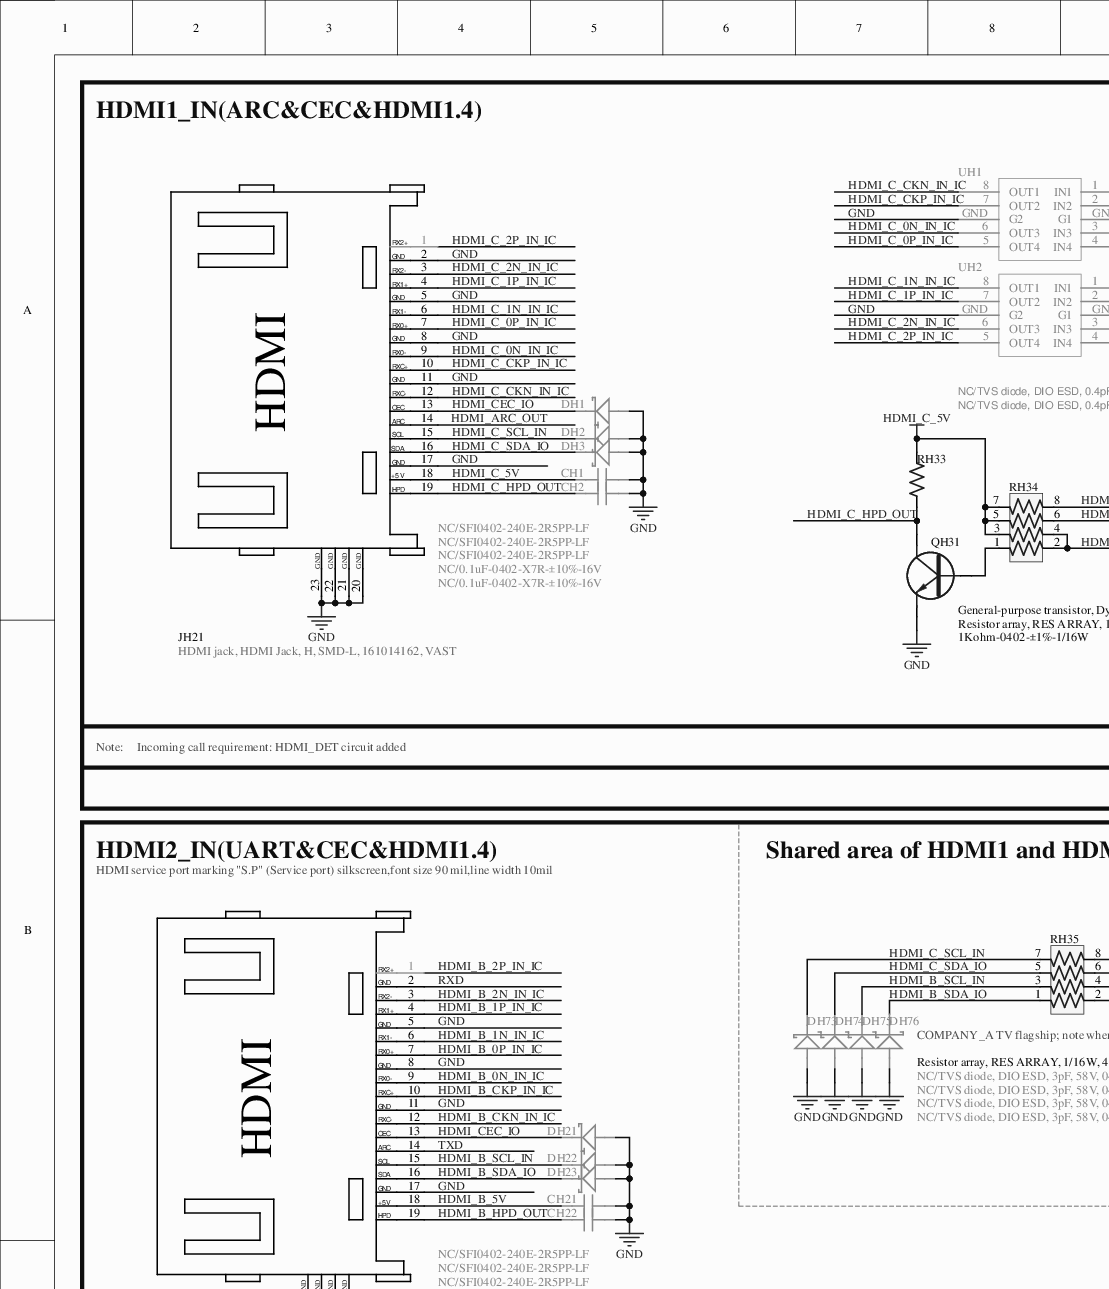
[diagram p0: MISC105950-40.SchDoc, top left]
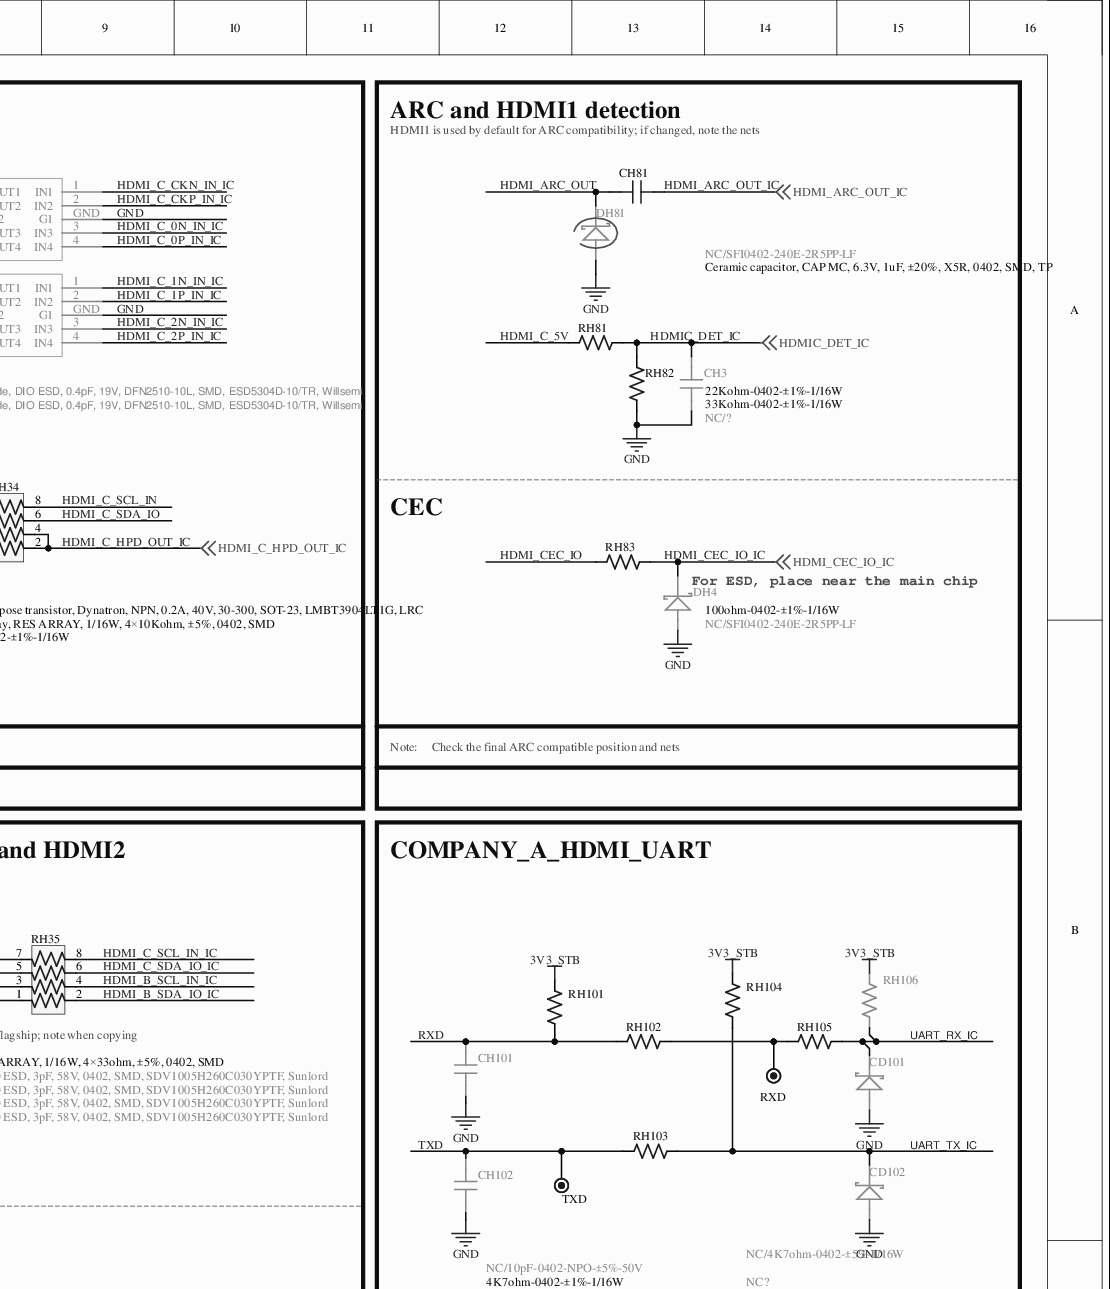
[diagram p1: MISC105950-40.SchDoc, top right]
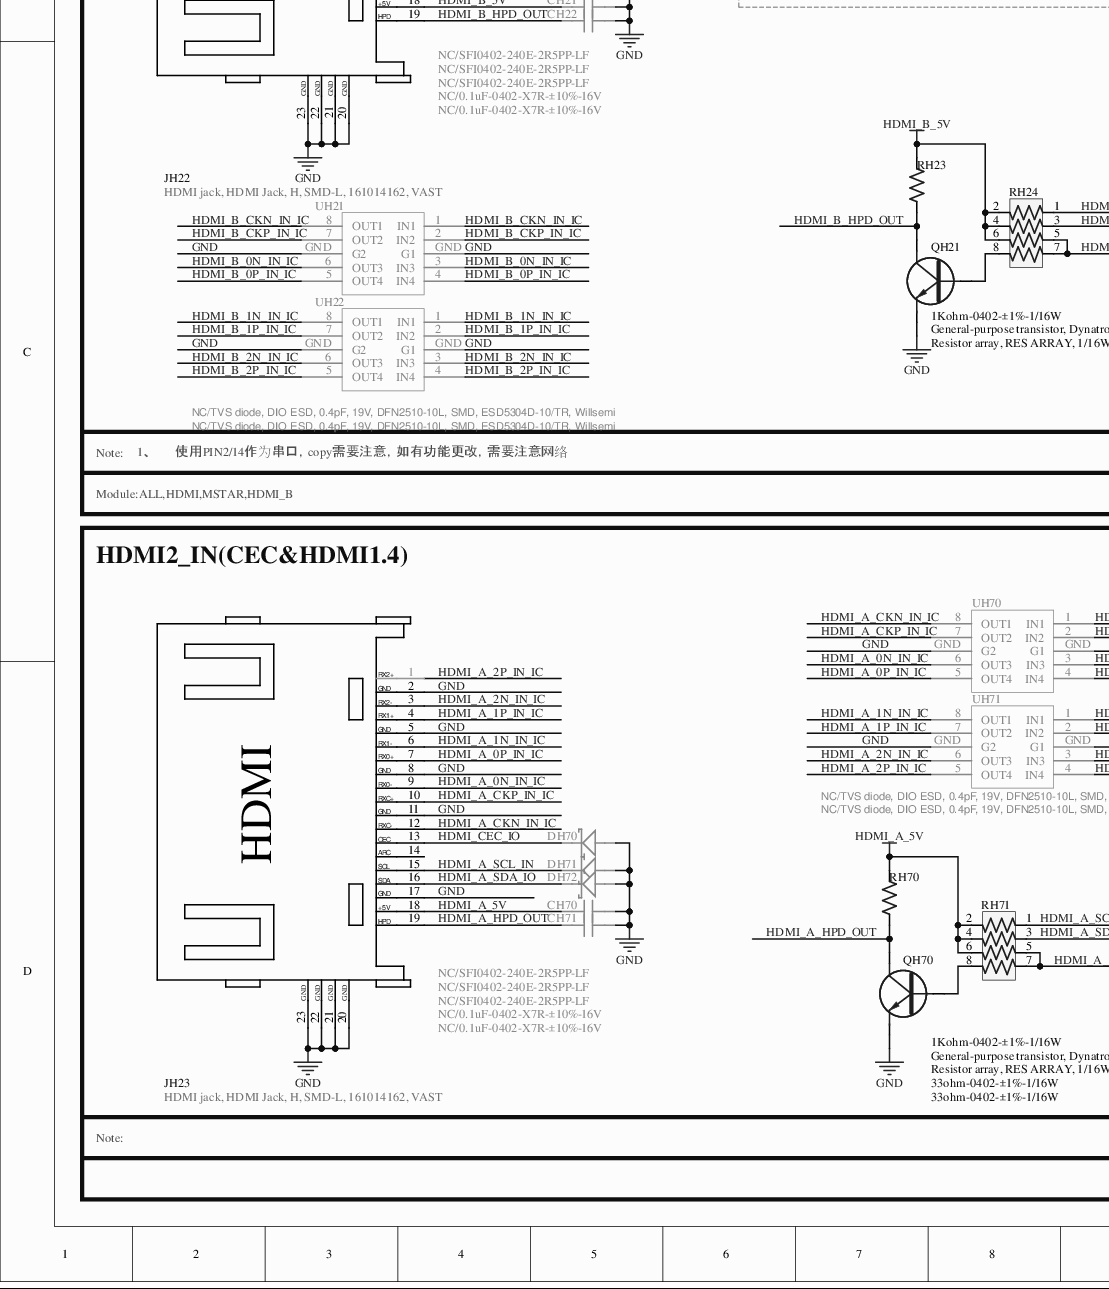
[diagram p2: MISC105950-40.SchDoc, bottom left]
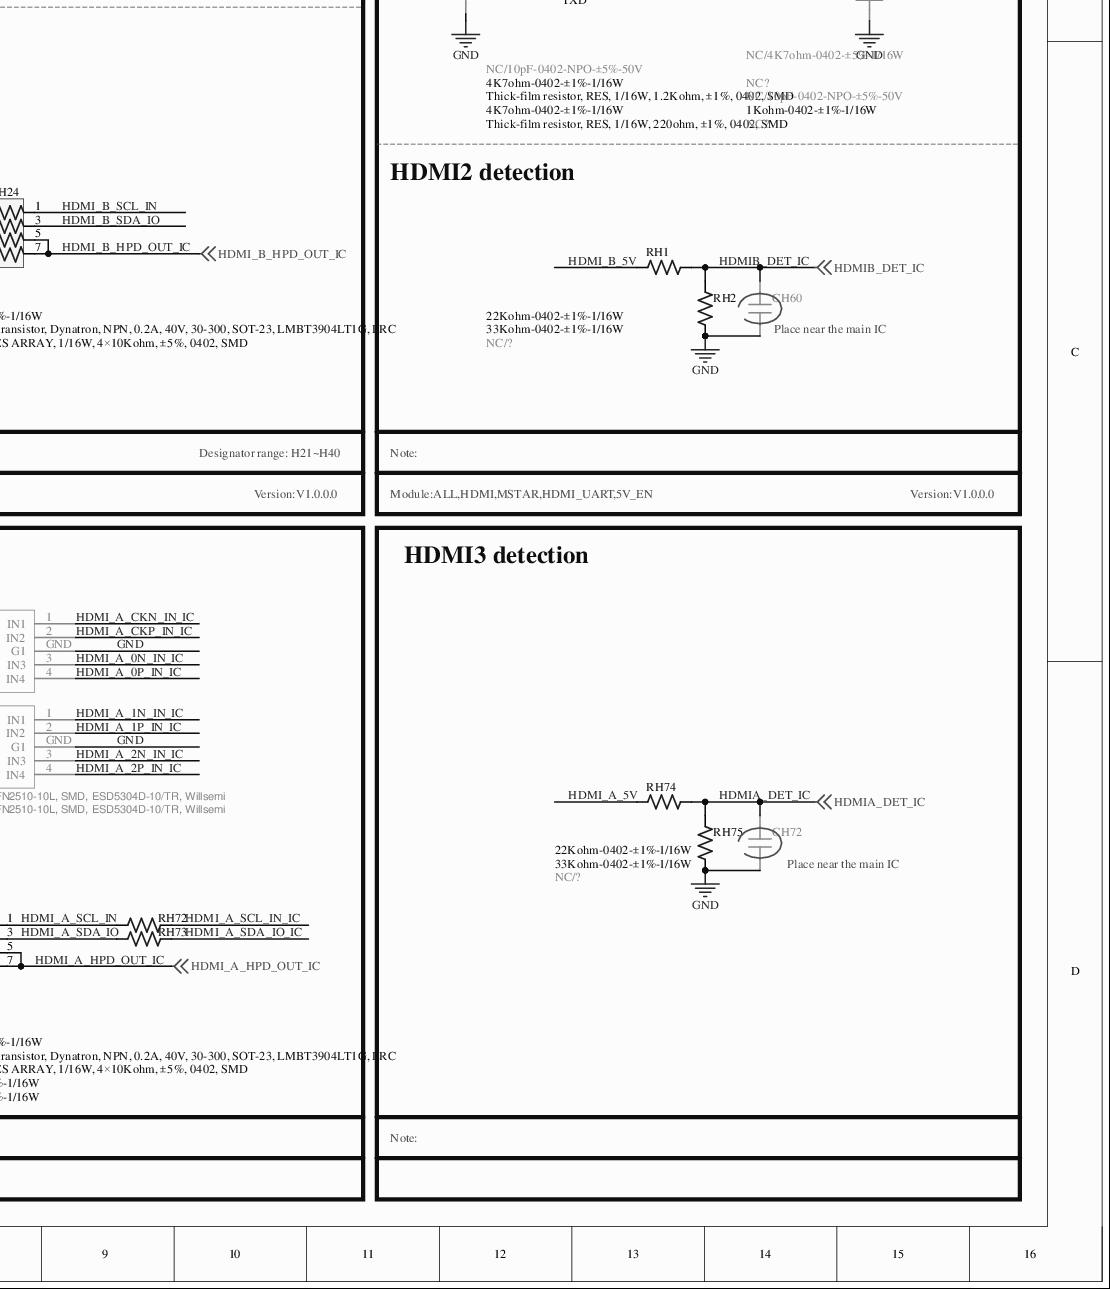
[diagram p3: MISC105950-40.SchDoc, bottom right]
# Altium project MISC105950-48.PrjPCB (part 6 of 8)

## Sheet MISC105950-40.SchDoc
size 393 x 459 mm

### Parts
CD101  NC?  [DIODE-S0402]
CD102  NC?  [DIODE-S0402]
CH1  NC/0.1uF-0402-X7R-±10%-16V  [C0402]
CH2  NC/0.1uF-0402-X7R-±10%-16V  [C0402]
CH3  NC/?  [C0402]
CH21  NC/0.1uF-0402-X7R-±10%-16V  [C0402]
CH22  NC/0.1uF-0402-X7R-±10%-16V  [C0402]
CH60  NC/?  [C0402]
CH70  NC/0.1uF-0402-X7R-±10%-16V  [C0402]
CH71  NC/0.1uF-0402-X7R-±10%-16V  [C0402]
CH72  NC/?  [C0402]
CH81  Ceramic capacitor, CAP MC, 6.3V, 1uF, ±20%, X5R, 0402, SMD, TP  [C0402]
CH101  NC/10pF-0402-NPO-±5%-50V  [C0402]
CH102  NC/10pF-0402-NPO-±5%-50V  [C0402]
DH1  NC/SFI0402-240E-2R5PP-LF  [DIODE-S0402]
DH2  NC/SFI0402-240E-2R5PP-LF  [DIODE-S0402]
DH3  NC/SFI0402-240E-2R5PP-LF  [DIODE-S0402]
DH4  NC/SFI0402-240E-2R5PP-LF  [DIODE-S0402]
DH21  NC/SFI0402-240E-2R5PP-LF  [DIODE-S0402]
DH22  NC/SFI0402-240E-2R5PP-LF  [DIODE-S0402]
DH23  NC/SFI0402-240E-2R5PP-LF  [DIODE-S0402]
DH70  NC/SFI0402-240E-2R5PP-LF  [DIODE-S0402]
DH71  NC/SFI0402-240E-2R5PP-LF  [DIODE-S0402]
DH72  NC/SFI0402-240E-2R5PP-LF  [DIODE-S0402]
DH73  NC/TVS diode, DIO ESD, 3pF, 58V, 0402, SMD, SDV1005H260C030YPTF, Sunlord  [DIODE-S0402]
DH74  NC/TVS diode, DIO ESD, 3pF, 58V, 0402, SMD, SDV1005H260C030YPTF, Sunlord  [DIODE-S0402]
DH75  NC/TVS diode, DIO ESD, 3pF, 58V, 0402, SMD, SDV1005H260C030YPTF, Sunlord  [DIODE-S0402]
DH76  NC/TVS diode, DIO ESD, 3pF, 58V, 0402, SMD, SDV1005H260C030YPTF, Sunlord  [DIODE-S0402]
DH81  NC/SFI0402-240E-2R5PP-LF  [DIODE-S0402]
JH21  HDMI jack, HDMI Jack, H, SMD-L, 161014162, VAST  [HDMI-HS-1]
JH22  HDMI jack, HDMI Jack, H, SMD-L, 161014162, VAST  [HDMI-HS-1]
JH23  HDMI jack, HDMI Jack, H, SMD-L, 161014162, VAST  [HDMI-HS-1]
QH21  General-purpose transistor, Dynatron, NPN, 0.2A, 40V, 30-300, SOT-23, LMBT3904LT1G, LRC  [SOT-23]
QH31  General-purpose transistor, Dynatron, NPN, 0.2A, 40V, 30-300, SOT-23, LMBT3904LT1G, LRC  [SOT-23]
QH70  General-purpose transistor, Dynatron, NPN, 0.2A, 40V, 30-300, SOT-23, LMBT3904LT1G, LRC  [SOT-23]
RH1  22Kohm-0402-±1%-1/16W  [R0402]
RH2  33Kohm-0402-±1%-1/16W  [R0402]
RH23  1Kohm-0402-±1%-1/16W  [R0402]
RH24  Resistor array, RES ARRAY, 1/16W, 4×10Kohm, ±5%, 0402, SMD  [RA0402]
RH33  1Kohm-0402-±1%-1/16W  [R0402]
RH34  Resistor array, RES ARRAY, 1/16W, 4×10Kohm, ±5%, 0402, SMD  [RA0402]
RH35  Resistor array, RES ARRAY, 1/16W, 4×33ohm, ±5%, 0402, SMD  [RA0402]
RH70  1Kohm-0402-±1%-1/16W  [R0402]
RH71  Resistor array, RES ARRAY, 1/16W, 4×10Kohm, ±5%, 0402, SMD  [RA0402]
RH72  33ohm-0402-±1%-1/16W  [R0402]
RH73  33ohm-0402-±1%-1/16W  [R0402]
RH74  22Kohm-0402-±1%-1/16W  [R0402]
RH75  33Kohm-0402-±1%-1/16W  [R0402]
RH81  22Kohm-0402-±1%-1/16W  [R0402]
RH82  33Kohm-0402-±1%-1/16W  [R0402]
RH83  100ohm-0402-±1%-1/16W  [R0402]
RH101  4K7ohm-0402-±1%-1/16W  [R0402]
RH102  Thick-film resistor, RES, 1/16W, 1.2Kohm, ±1%, 0402, SMD  [R0402]
RH103  1Kohm-0402-±1%-1/16W  [R0402]
RH104  4K7ohm-0402-±1%-1/16W  [R0402]
RH105  Thick-film resistor, RES, 1/16W, 220ohm, ±1%, 0402, SMD  [R0402]
RH106  NC/4K7ohm-0402-±5%-1/16W  [R0402]
RXD  (no value)  [TP]
TXD  (no value)  [TP]
UH1  NC/TVS diode, DIO ESD, 0.4pF, 19V, DFN2510-10L, SMD, ESD5304D-10/TR, Willsemi  [RCL0524P]
UH2  NC/TVS diode, DIO ESD, 0.4pF, 19V, DFN2510-10L, SMD, ESD5304D-10/TR, Willsemi  [RCL0524P]
UH21  NC/TVS diode, DIO ESD, 0.4pF, 19V, DFN2510-10L, SMD, ESD5304D-10/TR, Willsemi  [RCL0524P]
UH22  NC/TVS diode, DIO ESD, 0.4pF, 19V, DFN2510-10L, SMD, ESD5304D-10/TR, Willsemi  [RCL0524P]
UH70  NC/TVS diode, DIO ESD, 0.4pF, 19V, DFN2510-10L, SMD, ESD5304D-10/TR, Willsemi  [RCL0524P]
UH71  NC/TVS diode, DIO ESD, 0.4pF, 19V, DFN2510-10L, SMD, ESD5304D-10/TR, Willsemi  [RCL0524P]

### Blocks framed on the sheet
HDMI1_IN(ARC&CEC&HDMI1.4): CH1 CH2 DH1-DH3 JH21 QH31 RH33 RH34 UH1 UH2
HDMI2_IN(CEC&HDMI1.4): CH70 CH71 DH70-DH72 JH23 QH70 RH70-RH73 UH70 UH71
HDMI3 detection: CH72 RH74 RH75

### Nets
3V3_STB: RH101.2 RH104.2 RH106.2
GND: CD101.A CD102.A CH1.2 CH2.2 CH3.1 CH21.2 CH22.2 CH60.1 CH70.2 CH71.2 CH72.1 CH101.1 CH102.1 DH1.A DH2.A DH3.A DH4.A DH21.A DH22.A DH23.A DH70.A DH71.A DH72.A DH73.A DH74.A DH75.A DH76.A DH81.A JH21.2 JH21.5 JH21.8 JH21.11 JH21.17 JH21.20 JH21.21 JH21.22 JH21.23 JH22.5 JH22.8 JH22.11 JH22.17 JH22.20 JH22.21 JH22.22 JH22.23 JH23.2 JH23.5 JH23.8 JH23.11 JH23.17 JH23.20 JH23.21 JH23.22 JH23.23 QH21.E QH31.E QH70.E RH2.2 RH75.2 RH82.2 UH1.GND(G1) UH2.GND(G1) UH21.GND(G1) UH22.GND(G1) UH70.GND(G1) UH71.GND(G1)
HDMI_A_5V: CH70.1 JH23.18 RH70.2 RH71.2 RH71.4 RH71.6 RH74.2
HDMI_B_5V: CH21.1 JH22.18 RH1.2 RH23.2 RH24.2 RH24.4 RH24.6
HDMI_C_5V: CH1.1 JH21.18 RH33.2 RH34.3 RH34.5 RH34.7 RH81.2
HDMI_A_0N_IN_IC: JH23.9 UH70.3(IN3) UH70.6(OUT3)
HDMI_A_0P_IN_IC: JH23.7 UH70.4(IN4) UH70.5(OUT4)
HDMI_A_1N_IN_IC: JH23.6 UH71.1(IN1) UH71.8(OUT1)
HDMI_A_1P_IN_IC: JH23.4 UH71.2(IN2) UH71.7(OUT2)
HDMI_A_2N_IN_IC: JH23.3 UH71.3(IN3) UH71.6(OUT3)
HDMI_A_2P_IN_IC: JH23.1 UH71.4(IN4) UH71.5(OUT4)
HDMI_A_CKN_IN_IC: JH23.12 UH70.1(IN1) UH70.8(OUT1)
HDMI_A_CKP_IN_IC: JH23.10 UH70.2(IN2) UH70.7(OUT2)
HDMI_A_HPD_OUT: CH71.1 JH23.19 QH70.C RH70.1
HDMI_A_HPD_OUT_IC: RH71.5 RH71.7 ; off-sheet HDMI_A_HPD_OUT_IC
HDMI_A_SCL_IN: DH71.K JH23.15 RH71.1 RH72.1
HDMI_A_SCL_IN_IC: RH72.2
HDMI_A_SDA_IO: DH72.K JH23.16 RH71.3 RH73.1
HDMI_A_SDA_IO_IC: RH73.2
HDMI_ARC_OUT: CH81.1 DH81.K JH21.14
HDMI_ARC_OUT_IC: CH81.2 ; off-sheet HDMI_ARC_OUT_IC
HDMI_B_0N_IN_IC: JH22.9 UH21.3(IN3) UH21.6(OUT3)
HDMI_B_0P_IN_IC: JH22.7 UH21.4(IN4) UH21.5(OUT4)
HDMI_B_1N_IN_IC: JH22.6 UH22.1(IN1) UH22.8(OUT1)
HDMI_B_1P_IN_IC: JH22.4 UH22.2(IN2) UH22.7(OUT2)
HDMI_B_2N_IN_IC: JH22.3 UH22.3(IN3) UH22.6(OUT3)
HDMI_B_2P_IN_IC: JH22.1 UH22.4(IN4) UH22.5(OUT4)
HDMI_B_CKN_IN_IC: JH22.12 UH21.1(IN1) UH21.8(OUT1)
HDMI_B_CKP_IN_IC: JH22.10 UH21.2(IN2) UH21.7(OUT2)
HDMI_B_HPD_OUT: CH22.1 JH22.19 QH21.C RH23.1
HDMI_B_HPD_OUT_IC: RH24.5 RH24.7 ; off-sheet HDMI_B_HPD_OUT_IC
HDMI_B_SCL_IN: DH22.K DH75.K JH22.15 RH24.1 RH35.3
HDMI_B_SCL_IN_IC: RH35.4
HDMI_B_SDA_IO: DH23.K DH76.K JH22.16 RH24.3 RH35.1
HDMI_B_SDA_IO_IC: RH35.2
HDMI_C_0N_IN_IC: JH21.9 UH1.3(IN3) UH1.6(OUT3)
HDMI_C_0P_IN_IC: JH21.7 UH1.4(IN4) UH1.5(OUT4)
HDMI_C_1N_IN_IC: JH21.6 UH2.1(IN1) UH2.8(OUT1)
HDMI_C_1P_IN_IC: JH21.4 UH2.2(IN2) UH2.7(OUT2)
HDMI_C_2N_IN_IC: JH21.3 UH2.3(IN3) UH2.6(OUT3)
HDMI_C_2P_IN_IC: JH21.1 UH2.4(IN4) UH2.5(OUT4)
HDMI_C_CKN_IN_IC: JH21.12 UH1.1(IN1) UH1.8(OUT1)
HDMI_C_CKP_IN_IC: JH21.10 UH1.2(IN2) UH1.7(OUT2)
HDMI_C_HPD_OUT: CH2.1 JH21.19 QH31.C RH33.1
HDMI_C_HPD_OUT_IC: RH34.2 RH34.4 ; off-sheet HDMI_C_HPD_OUT_IC
HDMI_C_SCL_IN: DH2.K DH73.K JH21.15 RH34.8 RH35.7
HDMI_C_SCL_IN_IC: RH35.8
HDMI_C_SDA_IO: DH3.K DH74.K JH21.16 RH34.6 RH35.5
HDMI_C_SDA_IO_IC: RH35.6
HDMI_CEC_IO: DH1.K DH21.K DH70.K JH21.13 JH22.13 JH23.13 RH83.2
HDMI_CEC_IO_IC: DH4.K RH83.1 ; off-sheet HDMI_CEC_IO_IC
HDMIA_DET_IC: CH72.2 RH74.1 RH75.1 ; off-sheet HDMIA_DET_IC
HDMIB_DET_IC: CH60.2 RH1.1 RH2.1 ; off-sheet HDMIB_DET_IC
HDMIC_DET_IC: CH3.2 RH81.1 RH82.1 ; off-sheet HDMIC_DET_IC
RXD: CH101.2 JH22.2 RH101.1 RH102.1
TXD: CH102.2 JH22.14 RH103.1 TXD.1
UART_RX_IC: CD101.K RH105.2 RH106.1
UART_TX_IC: CD102.K RH103.2 RH104.1
NetQH21_B: QH21.B RH24.8
NetQH31_B: QH31.B RH34.1
NetQH70_B: QH70.B RH71.8
NetRH102_2: RH102.2 RH105.1 RXD.1

Not connected (* = marked no-connect by the designer): JH23 14*

### Notes on the sheet
- ARC and HDMI1 detection
- HDMI1 is used by default for ARC compatibility; if changed, note the nets
- CEC
- (near DH4) For ESD, place near the main chip
- Note:
- Incoming call requirement: HDMI_DET circuit added
- Check the final ARC compatible position and nets
- HDMI2_IN(UART&CEC&HDMI1.4)
- Shared area of HDMI1 and HDMI2
- COMPANY_A_HDMI_UART
- HDMI service port marking "S.P" (Service port) silkscreen,font size 90 mil,line width 10mil
- COMPANY_A TV flagship; note when copying
- HDMI2 detection
- (near CH60) Place near the main IC
- 1、COMPANY_A使用PIN2/14作为串口，copy需要注意，如有功能更改，需要注意网络
- Designator range: H21~H40
- Module:ALL,HDMI,MSTAR,HDMI_B
- Version:V1.0.0.0
- Module:ALL,HDMI,MSTAR,HDMI_UART,5V_EN
- (near CH72) Place near the main IC

### Library data of the parts
CD101 CD102 DH73-DH76 = AVLC18S02003-D
CH1-CH3 CH21 CH22 CH60 CH70-CH72 = 0.1uF-0402-X5R-±20%-16V-D
CH81 = 1uF-0402-X5R-±20%-6.3V-D
CH101 CH102 = 220pF-0402-X7R-±10%-50V-D
DH1-DH4 DH21-DH23 DH70-DH72 DH81 = 004.005.0000315-D: TVS diode, DIO ESD, 2.5pF, 200V, 0402, SMD, SFI0402-240E-2R5PP-LF, SFI-D
JH21-JH23 = 161031041(外壳SPCC)-D: CN-HDMI-horizontal-#-#
QH21 QH31 QH70 = 004.006.0000007-D: General-purpose transistor, Dynatron, NPN, 0.2A, 40V, 60-300, SOT-23, KMBT3904, KEXIN-D
RH1 RH74 RH81 = 22Kohm-0402-±5%-1/16W-D
RH2 RH75 RH82 = 33Kohm-0402-±5%-1/16W-D
RH23 RH33 RH70 = 1Kohm-0402-±5%-1/16W-D
RH24 RH34 RH35 RH71 = 4*100ohm-0402-±5%-1/16W-D
RH72 RH73 = 33ohm-0402-±5%-1/16W-D
RH83 = 004.002.0000568-D: Thick-film resistor, RES, 1/16W, 100ohm, ±5%, 0402, SMD-D
RH101-RH106 = 68ohm-0402-±5%-1/16W-D
RXD TXD = TEST
UH1 UH2 UH21 UH22 UH70 UH71 = ULC0524P-D: RCLAMP0524J

## Sheet MISC105950-41.SchDoc
size 292 x 218 mm
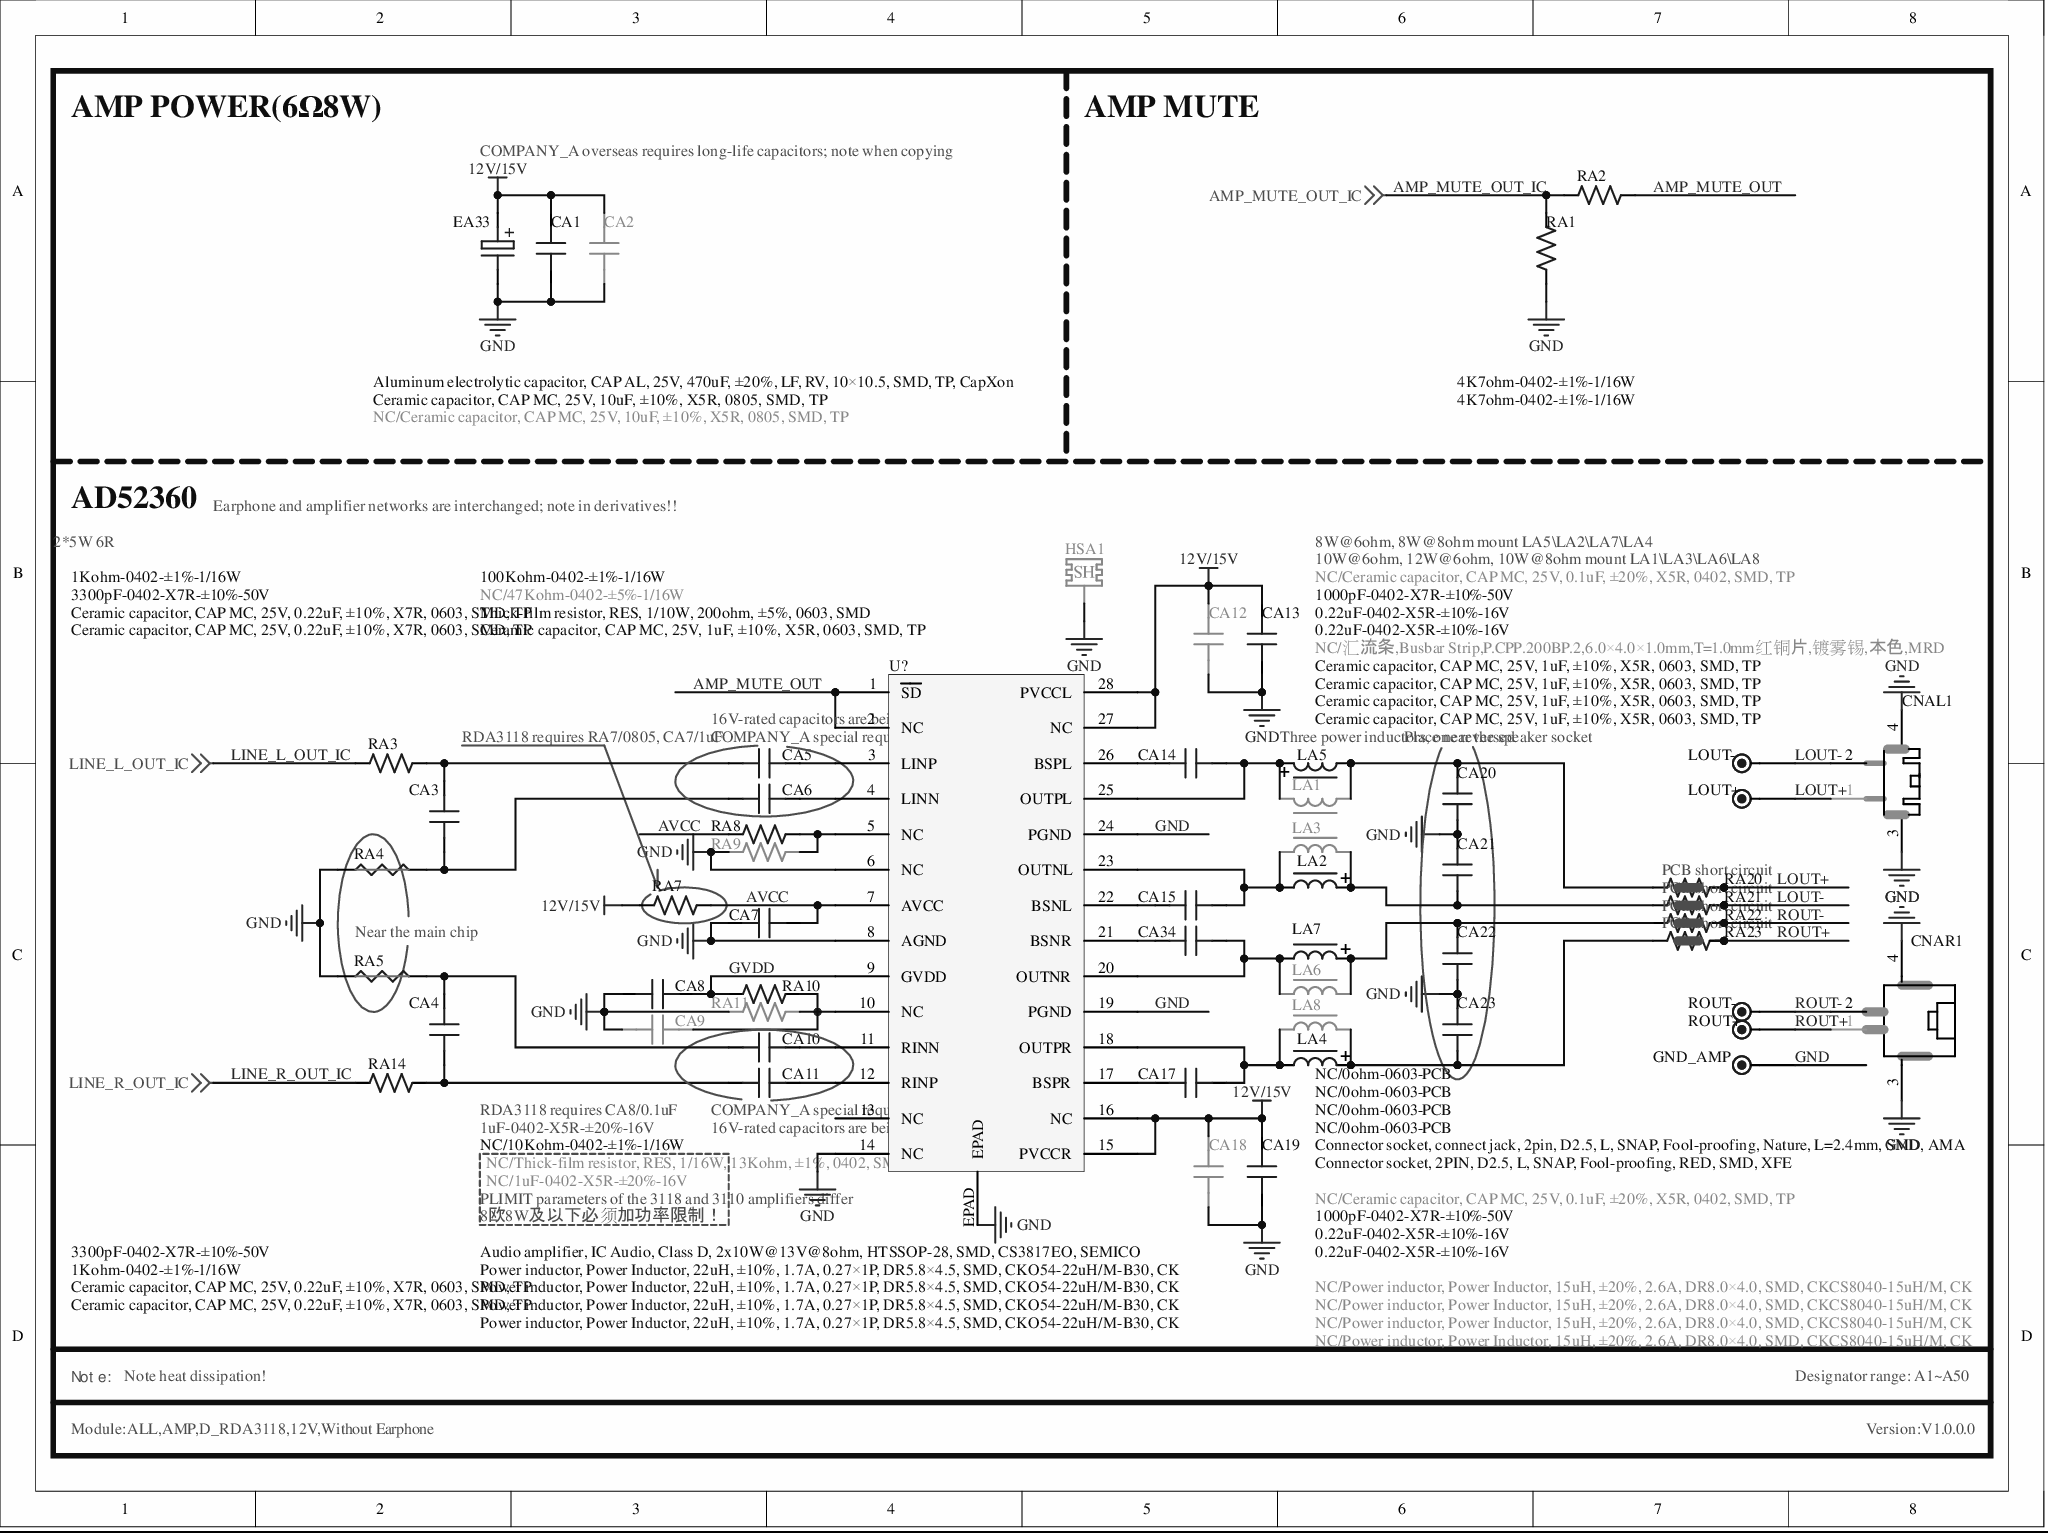
[diagram p4: MISC105950-41.SchDoc]

### Parts
CA1  Ceramic capacitor, CAP MC, 25V, 10uF, ±10%, X5R, 0805, SMD, TP  [C0805]
CA2  NC/Ceramic capacitor, CAP MC, 25V, 10uF, ±10%, X5R, 0805, SMD, TP  [C0805]
CA3  3300pF-0402-X7R-±10%-50V  [C0402]
CA4  3300pF-0402-X7R-±10%-50V  [C0402]
CA5  Ceramic capacitor, CAP MC, 25V, 0.22uF, ±10%, X7R, 0603, SMD, TP  [C0603]
CA6  Ceramic capacitor, CAP MC, 25V, 0.22uF, ±10%, X7R, 0603, SMD, TP  [C0603]
CA7  Ceramic capacitor, CAP MC, 25V, 1uF, ±10%, X5R, 0603, SMD, TP  [C0603]
CA8  1uF-0402-X5R-±20%-16V  [C0402]
CA9  NC/1uF-0402-X5R-±20%-16V  [C0402]
CA10  Ceramic capacitor, CAP MC, 25V, 0.22uF, ±10%, X7R, 0603, SMD, TP  [C0603]
CA11  Ceramic capacitor, CAP MC, 25V, 0.22uF, ±10%, X7R, 0603, SMD, TP  [C0603]
CA12  NC/Ceramic capacitor, CAP MC, 25V, 0.1uF, ±20%, X5R, 0402, SMD, TP  [C0402]
CA13  1000pF-0402-X7R-±10%-50V  [C0402]
CA14  0.22uF-0402-X5R-±10%-16V  [C0402]
CA15  0.22uF-0402-X5R-±10%-16V  [C0402]
CA17  0.22uF-0402-X5R-±10%-16V  [C0402]
CA18  NC/Ceramic capacitor, CAP MC, 25V, 0.1uF, ±20%, X5R, 0402, SMD, TP  [C0402]
CA19  1000pF-0402-X7R-±10%-50V  [C0402]
CA20  Ceramic capacitor, CAP MC, 25V, 1uF, ±10%, X5R, 0603, SMD, TP  [C0603]
CA21  Ceramic capacitor, CAP MC, 25V, 1uF, ±10%, X5R, 0603, SMD, TP  [C0603]
CA22  Ceramic capacitor, CAP MC, 25V, 1uF, ±10%, X5R, 0603, SMD, TP  [C0603]
CA23  Ceramic capacitor, CAP MC, 25V, 1uF, ±10%, X5R, 0603, SMD, TP  [C0603]
CA34  0.22uF-0402-X5R-±10%-16V  [C0402]
CNAL1  Connector socket, connect jack, 2pin, D2.5, L, SNAP, Fool-proofing, Nature, L=2.4mm, SMD, AMA  [SIP2H/2.5S-4]
CNAR1  Connector socket, 2PIN, D2.5, L, SNAP, Fool-proofing, RED, SMD, XFE  [SIP2H/2.5S-3]
EA33  Aluminum electrolytic capacitor, CAP AL, 25V, 470uF, ±20%, LF, RV, 10×10.5, SMD, TP, CapXon  [EC(10*10.5)-S]
GND_AMP  DM0  [TP]  (value not drawn)
HSA1  NC/汇流条,Busbar Strip,P.CPP.200BP.2,6.0×4.0×1.0mm,T=1.0mm红铜片,镀雾锡,本色,MRD  [HL030]
LA1  NC/Power inductor, Power Inductor, 15uH, ±20%, 2.6A, DR8.0×4.0, SMD, CKCS8040-15uH/M, CK  [L(8*4.2)-S]
LA2  Power inductor, Power Inductor, 22uH, ±10%, 1.7A, 0.27×1P, DR5.8×4.5, SMD, CKO54-22uH/M-B30, CK  [L(5.8*4.5)-S-3]
LA3  NC/Power inductor, Power Inductor, 15uH, ±20%, 2.6A, DR8.0×4.0, SMD, CKCS8040-15uH/M, CK  [L(8*4.2)-S]
LA4  Power inductor, Power Inductor, 22uH, ±10%, 1.7A, 0.27×1P, DR5.8×4.5, SMD, CKO54-22uH/M-B30, CK  [L(5.8*4.5)-S-3]
LA5  Power inductor, Power Inductor, 22uH, ±10%, 1.7A, 0.27×1P, DR5.8×4.5, SMD, CKO54-22uH/M-B30, CK  [L(5.8*4.5)-S-3]
LA6  NC/Power inductor, Power Inductor, 15uH, ±20%, 2.6A, DR8.0×4.0, SMD, CKCS8040-15uH/M, CK  [L(8*4.2)-S]
LA7  Power inductor, Power Inductor, 22uH, ±10%, 1.7A, 0.27×1P, DR5.8×4.5, SMD, CKO54-22uH/M-B30, CK  [L(5.8*4.5)-S-3]
LA8  NC/Power inductor, Power Inductor, 15uH, ±20%, 2.6A, DR8.0×4.0, SMD, CKCS8040-15uH/M, CK  [L(8*4.2)-S]
LOUT+  DM0  [TP]  (value not drawn)
LOUT-  DM0  [TP]  (value not drawn)
RA1  4K7ohm-0402-±1%-1/16W  [R0402]
RA2  4K7ohm-0402-±1%-1/16W  [R0402]
RA3  1Kohm-0402-±1%-1/16W  [R0402]
RA4  NC/?  [GND]  (value not drawn)
RA5  NC/?  [GND]  (value not drawn)
RA7  Thick-film resistor, RES, 1/10W, 200ohm, ±5%, 0603, SMD  [R0603]
RA8  100Kohm-0402-±1%-1/16W  [R0402]
RA9  NC/47Kohm-0402-±5%-1/16W  [R0402]
RA10  NC/10Kohm-0402-±1%-1/16W  [R0402]
RA11  NC/Thick-film resistor, RES, 1/16W, 13Kohm, ±1%, 0402, SMD  [R0402]
RA14  1Kohm-0402-±1%-1/16W  [R0402]
RA20  NC/0ohm-0603-PCB  [R0603SC]
RA21  NC/0ohm-0603-PCB  [R0603SC]
RA22  NC/0ohm-0603-PCB  [R0603SC]
RA23  NC/0ohm-0603-PCB  [R0603SC]
ROUT+  DM0  [TP]  (value not drawn)
ROUT-  DM0  [TP]  (value not drawn)
U?  Audio amplifier, IC Audio, Class D, 2x10W@13V@8ohm, HTSSOP-28, SMD, CS3817EO, SEMICO  [SSOP28/0.65-5]

### Nets
12V/15V: CA1.2 CA2.2 CA12.2 CA13.2 CA18.2 CA19.2 EA33.1 RA7.1 U?.15(PVCCR) U?.16(NC) U?.27(NC) U?.28(PVCCL)
GND: CA1.1 CA2.1 CA7.1 CA8.1 CA9.1 CA12.1 CA13.1 CA18.1 CA19.1 CA20.1 CA21.2 CA22.1 CA23.2 CNAL1.3 CNAL1.4 CNAR1.3 CNAR1.4 EA33.2 GND_AMP.1 HSA1.1 RA1.2 RA4.JP_2K RA5.JP_2K RA9.1 RA11.1 U?.6(NC) U?.8(AGND) U?.14(NC) U?.19(PGND) U?.24(PGND) U?.EPAD
AMP_MUTE_OUT: RA2.1 U?.1(~{SD}) U?.2(NC)
AMP_MUTE_OUT_IC: RA1.1 RA2.2 ; off-sheet AMP_MUTE_OUT_IC
AVCC: CA7.2 RA7.2 RA8.1 U?.7(AVCC)
GVDD: CA8.2 RA10.1 U?.9(GVDD)
LINE_L_OUT_IC: RA3.1 ; off-sheet LINE_L_OUT_IC
LINE_R_OUT_IC: RA14.1 ; off-sheet LINE_R_OUT_IC
LOUT+: CNAL1.1 LOUT+.1 RA20.2 RA20.3
LOUT-: CNAL1.2 LOUT-.1 RA21.2 RA21.3
ROUT+: CNAR1.1 RA23.2 RA23.3 ROUT+.1
ROUT-: CNAR1.2 RA22.2 RA22.3 ROUT-.1
NetCA3_1: CA3.1 CA6.1 RA4.JP_1K
NetCA3_2: CA3.2 CA5.1 RA3.2
NetCA4_1: CA4.1 CA11.1 RA14.2
NetCA4_2: CA4.2 CA10.1 RA5.JP_1K
NetCA5_2: CA5.2 U?.3(LINP)
NetCA6_2: CA6.2 U?.4(LINN)
NetCA9_2: CA9.2 RA10.2 RA11.2 U?.10(NC)
NetCA10_2: CA10.2 U?.11(RINN)
NetCA11_2: CA11.2 U?.12(RINP)
NetCA14_1: CA14.1 U?.26(BSPL)
NetCA14_2: CA14.2 LA1.2 LA5.S U?.25(OUTPL)
NetCA15_1: CA15.1 U?.22(BSNL)
NetCA15_2: CA15.2 LA2.F LA3.1 U?.23(OUTNL)
NetCA17_1: CA17.1 U?.17(BSPR)
NetCA17_2: CA17.2 LA4.F LA8.1 U?.18(OUTPR)
NetCA20_2: CA20.2 LA1.1 LA5.F RA20.1
NetCA21_1: CA21.1 LA2.S LA3.2 RA21.1
NetCA22_2: CA22.2 LA6.2 LA7.S RA22.1
NetCA23_1: CA23.1 LA4.S LA8.2 RA23.1
NetCA34_1: CA34.1 U?.21(BSNR)
NetCA34_2: CA34.2 LA6.1 LA7.F U?.20(OUTNR)
NetRA8_2: RA8.2 RA9.2 U?.5(NC)

Not connected (* = marked no-connect by the designer): U? 13(NC)*

### Notes on the sheet
- AMP POWER(6Ω8W)
- AMP MUTE
- COMPANY_A overseas requires long-life capacitors; note when copying
- 2*5W 6R
- AD52360
- Earphone and amplifier networks are interchanged; note in derivatives!!
- 8W@6ohm, 8W@8ohm mount LA5\LA2\LA7\LA4
- 10W@6ohm, 12W@6ohm, 10W@8ohm mount LA1\LA3\LA6\LA8
- (near CA5) RDA3118 requires RA7/0805, CA7/1uF
- (near U?) COMPANY_A special requirement
- (near U?) 16V-rated capacitors are being phased out
- Three power inductors, one reversed
- (near CA20) Place near the speaker socket
- Near the main chip
- RDA3118 requires CA8/0.1uF
- (near U?) PLIMIT parameters of the 3118 and 3110 amplifiers differ
- 8欧8W及以下必须加功率限制！
- Note:
- Note heat dissipation!
- Designator range: A1~A50
- Module:ALL,AMP,D_RDA3118,12V,Without Earphone
- Version:V1.0.0.0

### Library data of the parts
CA1 CA2 = 004.003.0000386-D: Ceramic capacitor, CAP MC, 16V, 10uF, ±20%, X5R, 0805, SMD, TP-D
CA3 CA4 = 004.003.0000549-D: Ceramic capacitor, CAP MC, 50V, 3300pF, ±10%, X7R, 0402, SMD, TP-D
CA5 CA6 CA10 CA11 = 004.003.0000400-D: Ceramic capacitor, CAP MC, 16V, 0.22uF, ±10%, X5R, 0603, SMD, TP-D
CA7 CA20-CA23 = 1uF-0603-X7R-±10%-10V-D
CA8 CA12 CA18 = 004.003.0000403-D: Ceramic capacitor, CAP MC, 16V, 0.1uF, ±20%, X5R, 0402, SMD, TP-D
CA9 = 004.003.0000402-D: Ceramic capacitor, CAP MC, 16V, 1uF, ±20%, X5R, 0402, SMD, TP-D
CA13 CA19 = 004.003.0000503-D: Ceramic capacitor, CAP MC, 50V, 1000pF, ±10%, X7R, 0402, SMD, TP-D
CA14 CA15 CA17 CA34 = 004.003.0000398-D: Ceramic capacitor, CAP MC, 16V, 0.22uF, ±20%, X5R, 0402, SMD, TP-D
CNAL1 = XXX.XXX.0001786-D: Connector socket, connect jack, 2pin, D2.5, L, SNAP, Fool-proofing, Nature, L=2.4mm, SMD, AMA-D
CNAR1 = 连接插座,2PIN,D2.5,L,SNAP,Fool-proofing,RED,SMD,XFE-D
EA33 = 铝电解电容,CAP AL,100V,33uF,±20%,LF,RV,10×10.5,SMD,TP,CapXon-D: Electrolytic
GND_AMP LOUT+ LOUT- ROUT+ ROUT- = TEST
HSA1 = 17.5×14.5×0.5-本色-Cu-MRD-D: Heatsink
LA1 LA3 LA6 LA8 = 004.004.0000054-D: Power inductor, Power Inductor, 15uH, ±20%, 2.60A, DR8.0×4.0, SMD, SWPA8040S150MT, Sunlord-D; Text Field1: 20; Text Field2: 40
LA2 LA4 LA5 LA7 = SMD5845-220M-03-1-HLY-D
RA1 RA2 = 004.002.0000689-D: Thick-film resistor, RES, 1/16W, 4.7Kohm, ±5%, 0402, SMD-D
RA3 RA14 = 004.002.0000572-D: Thick-film resistor, RES, 1/16W, 1Kohm, ±5%, 0402, SMD-D
RA4 RA5 = GND: Manufacturer: Panasonic; Part Number: ERJ3GEYJ473V; Right: 20; Bottom: 30; CLASS: Discrete; Comments: Digikey
RA7 = 004.002.0000200-D: Thick-film resistor, RES, 1/10W, 10Kohm, ±1%, 0603, SMD-D
RA8 = 004.002.0000579-D: Thick-film resistor, RES, 1/16W, 100Kohm, ±5%, 0402, SMD-D
RA9 = 004.002.0000691-D: Thick-film resistor, RES, 1/16W, 47Kohm, ±5%, 0402, SMD-D
RA10 = 004.002.0000575-D: Thick-film resistor, RES, 1/16W, 10Kohm, ±1%, 0402, SMD-D
RA11 = 004.002.0000602-D: Thick-film resistor, RES, 1/16W, 15Kohm, ±1%, 0402, SMD-D
RA20-RA23 = 0ohm-0603-PCB-D
U? = 004.012.0000328-D: Audio amplifier, IC Audio, Class D, 2x10W@13V@8ohm, HTSSOP-28, SMD, CS3817EO, SEMICO-D